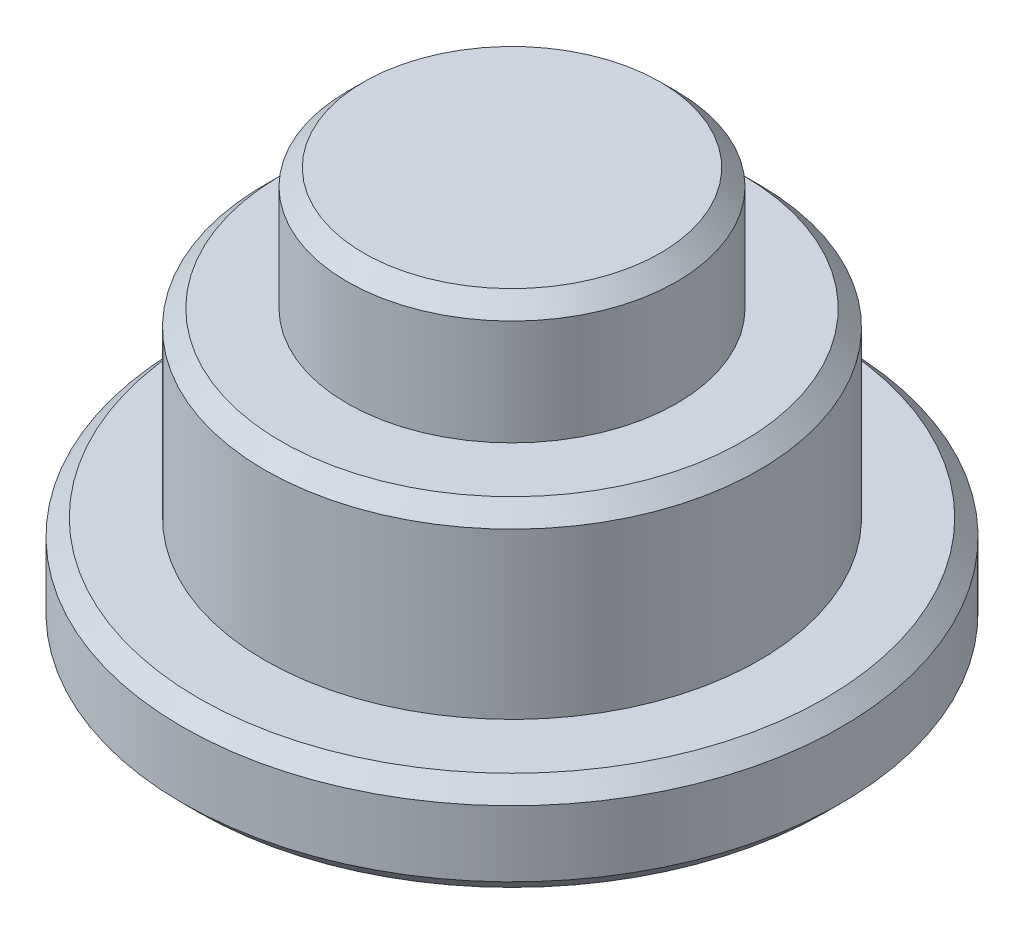
from build123d import *

# Parameters (mm, degrees)
CHAMFER1_SIZE = 0.5


with BuildPart() as part:
    # Sketch1 → Revolve1 (revolve)
    with BuildSketch(Plane.XY, mode=Mode.PRIVATE) as revolve1_sk:
        Polygon((131.66284067, -334.3040125), (131.66284067, -338.0040125), (129.16284067, -338.0040125), (129.16284067, -343.5040125), (126.66284067, -343.5040125), (126.66284067, -346.5040125), (136.66284067, -346.5040125), (136.66284067, -334.3040125), align=None)
    revolve(revolve1_sk.sketch.rotate(Axis((136.66284067, -346.5040125, 0), (0, 1, 0)), 270), axis=Axis((136.66284067, -346.5040125, 0), (0, 1, 0)))

    # Chamfer1
    chamfer1_edges = [part.edges().sort_by_distance(p)[0] for p in [
        (136.66284067, -334.3040125, 5),
        (136.66284067, -346.5040125, 10),
        (136.66284067, -343.5040125, 10),
        (136.66284067, -338.0040125, 7.5),
    ]]
    chamfer(chamfer1_edges, length=CHAMFER1_SIZE)


solid = part.part
